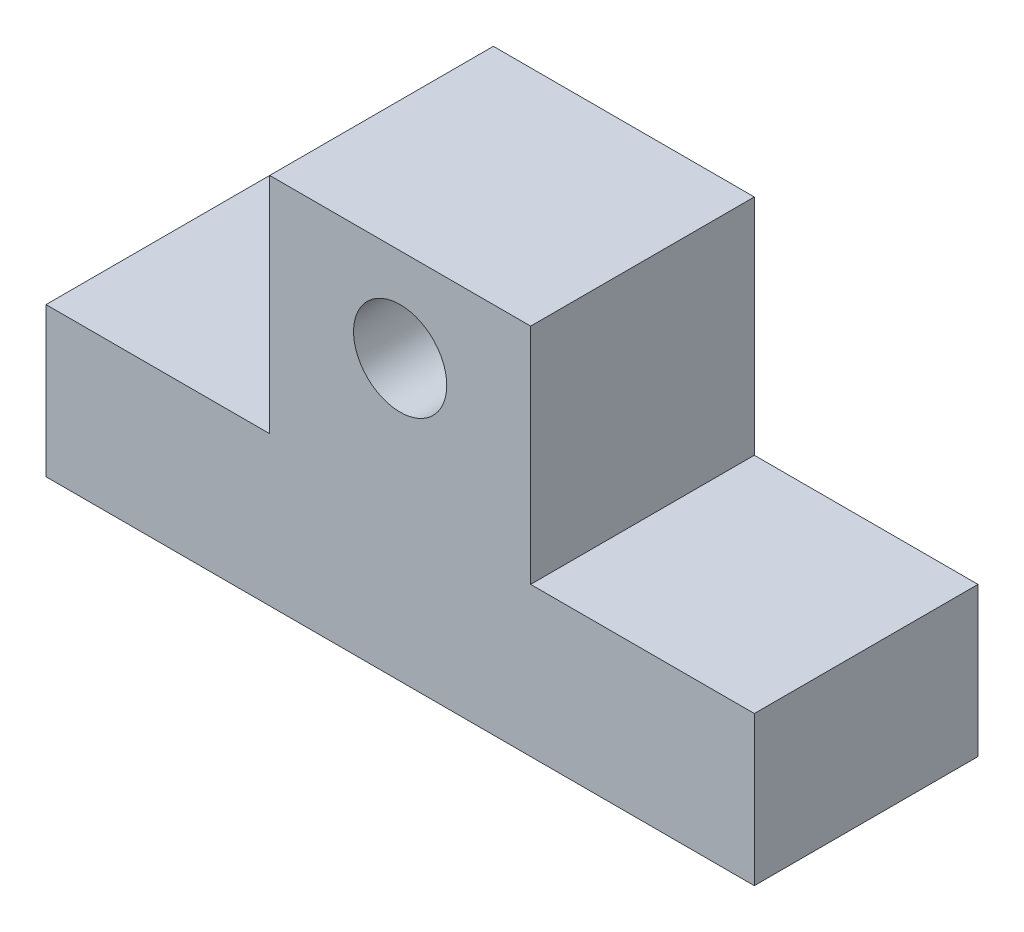
from build123d import *

# Parameters (mm, degrees)
EXTRUDE_1_DEPTH    = 6
HOLE_WIZARD_M6_1_D = 5


with BuildPart() as part:
    # 草图1 → 凸台-拉伸1 (new, symmetric)
    with BuildSketch(Plane.XY):
        Polygon((0, 0), (-7, 0), (-7, -12), (-19, -12), (-19, -20), (19, -20), (19, -12), (7, -12), (7, 0), align=None)
    extrude(amount=EXTRUDE_1_DEPTH, both=True)

    # M6 螺纹孔1 (through all)
    with Locations(Plane(origin=(0, -5, 6), x_dir=(1, 0, 0), z_dir=(0, 0, 1))):
        with Locations((0, 0)):
            Hole(HOLE_WIZARD_M6_1_D / 2)


solid = part.part
